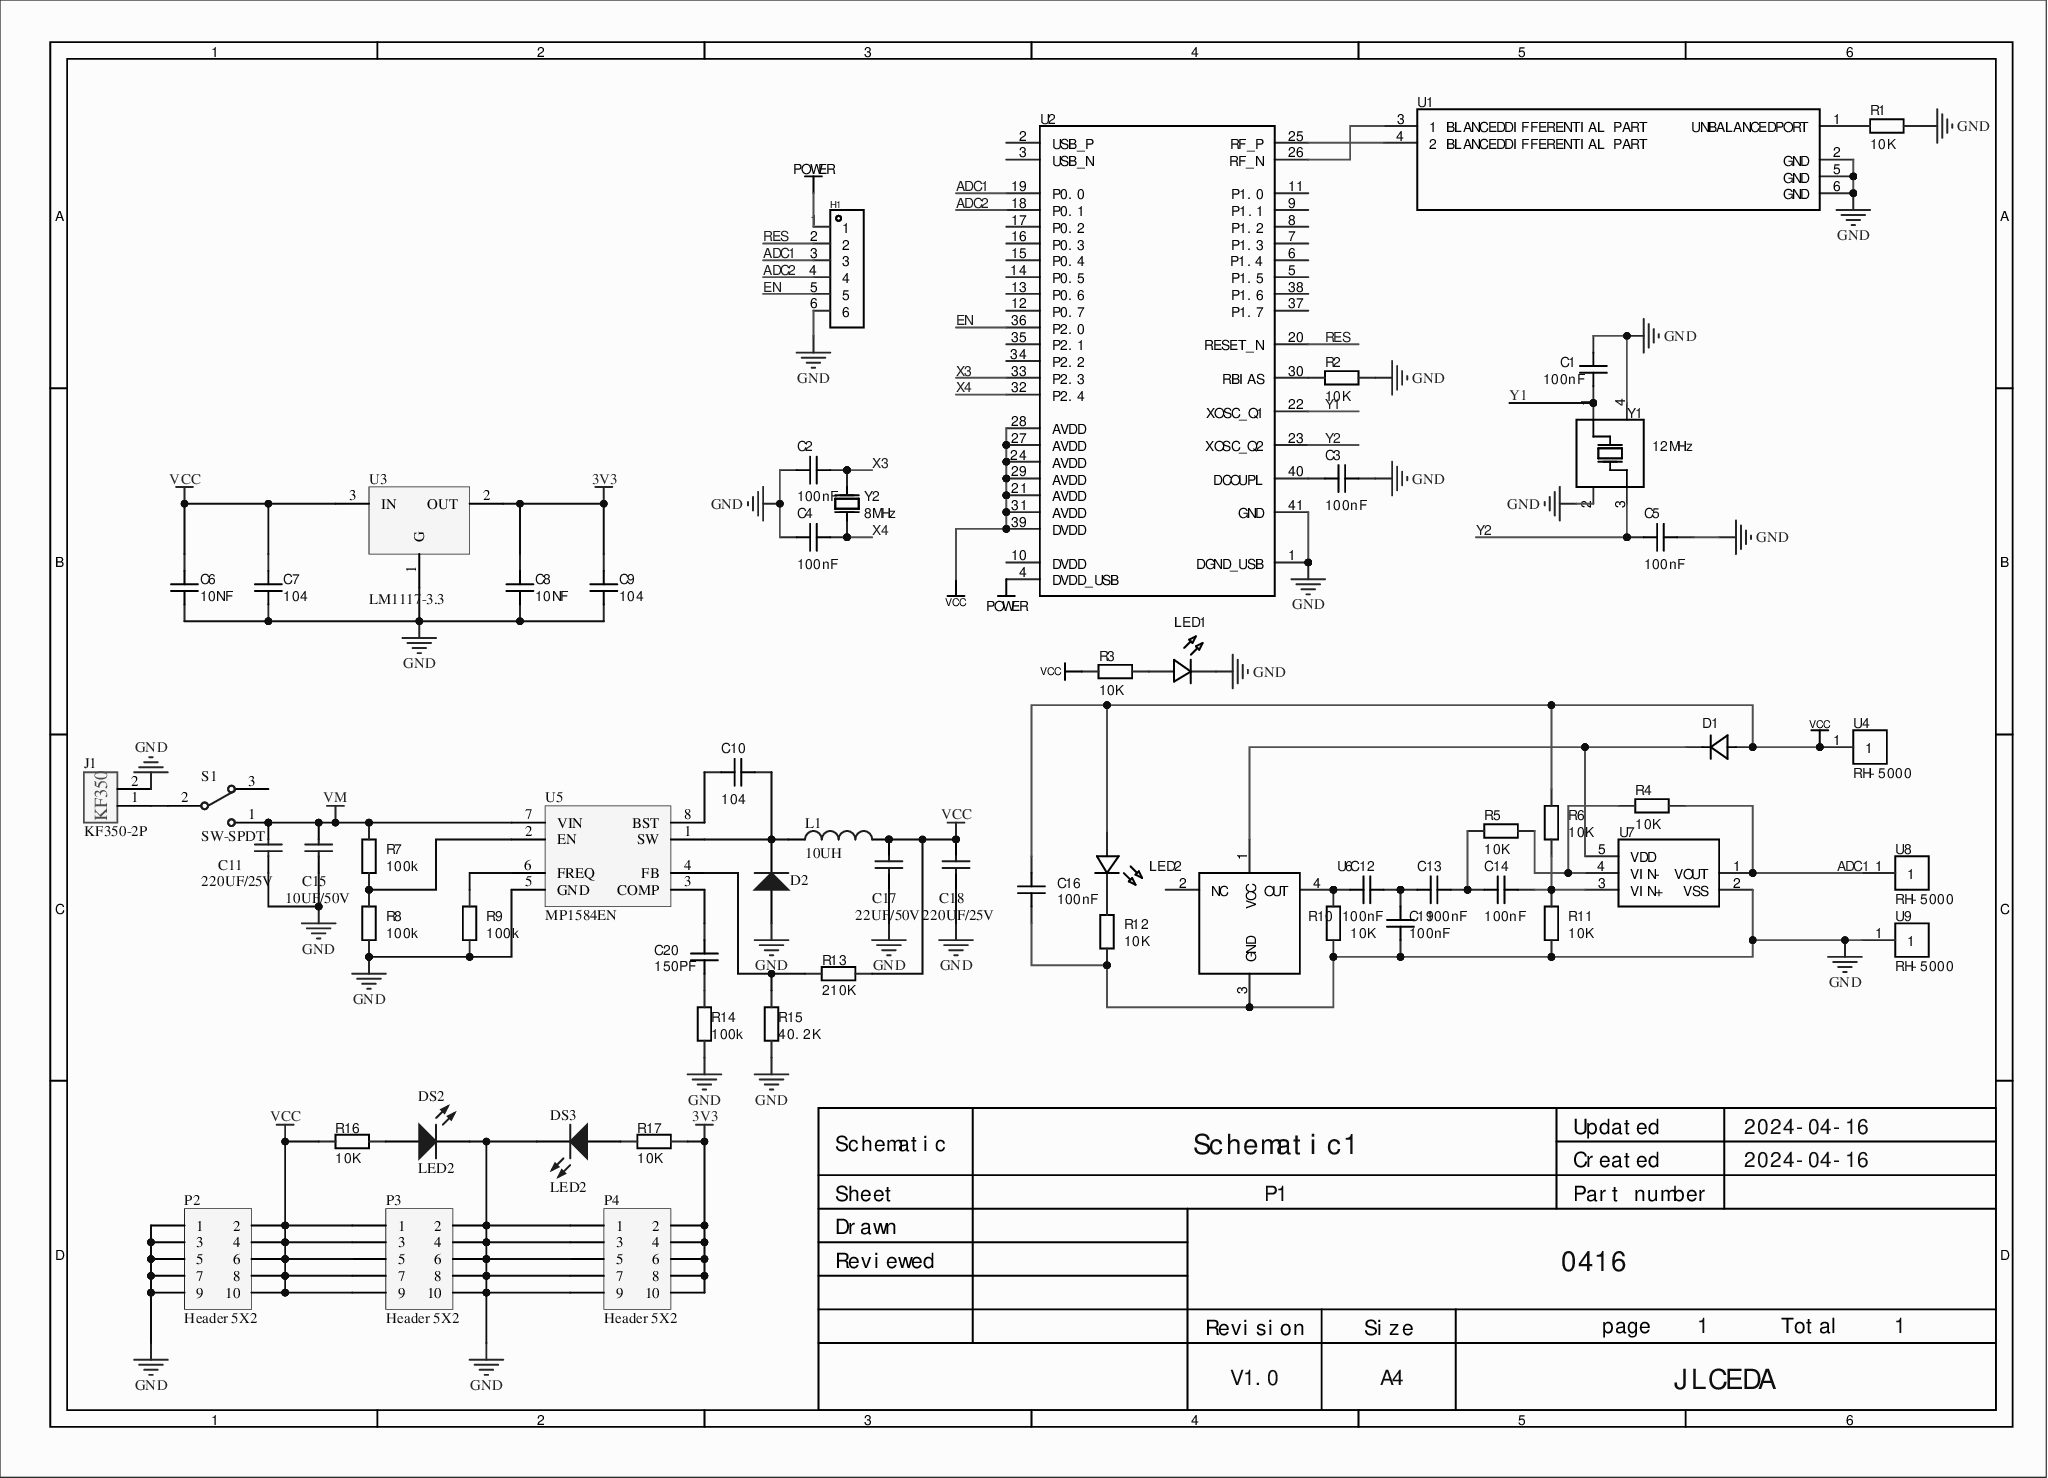
[diagram p0: MISC80555-2.SchDoc]
# Altium project MISC80555-3.PrjPcb
1 sheet, 61 parts. Net scope: global (net labels, ports and power ports of the same name join across sheets).
Board file: MISC80555.PcbDoc

## Sheet MISC80555-2.SchDoc
size 309 x 223 mm; Symbol: Sheet-Symbol_A4; Device: Sheet-Symbol_A4; @Page Name: P1; @Create Date: 2024-04-16; @Page Count: 1; @Page No: 1; @Project Name: 0416; @Schematic Name: Schematic1; @Update Date: 2024-04-16; Company: JLCEDA; Page Size: A4; Version: V1.0

### Parts
C1  100nF  [C0603]
C2  100nF  [C0603]
C3  100nF  [C0603]
C4  100nF  [C0603]
C5  100nF  [C0603]
C6  Name: 10NF  [C0603]  (hidden comment: 100nF)
C7  Name: 104  [C0603]  (hidden comment: 100nF)
C8  Name: 10NF  [C0603]  (hidden comment: 100nF)
C9  Name: 104  [C0603]  (hidden comment: 100nF)
C10  Name: 104  [C0603]  (hidden comment: 100nF)
C11  220UF/25V  [贴片电容]
C12  100nF  [C0603]
C13  100nF  [C0603]
C14  100nF  [C0603]
C15  10UF/50V  [贴片电容]
C16  100nF  [C0603]
C17  22UF/50V  [贴片电容]
C18  220UF/25V  [贴片电容]
C19  100nF  [C0603]
C20  Name: 150PF  [C0603]  (hidden comment: 100nF)
D1  D_1N4007A  [3.2X1.6X1.1]  (value not drawn)
D2  Diode BAS16  [3.2X1.6X1.1]  (value not drawn)
DS2  LED2  [my0603LED]
DS3  LED2  [my0603LED]
H1  HDR-F_2.54_1x6P  [HDR1X6]  (value not drawn)
J1  KF350-2P  [KF350-2P]
L1  10UH  [0402-A]
LED1  LED_0603-R  [my0603LED]  (value not drawn)
LED2  LED_0603-R  [my0603LED]  (value not drawn)
P2  Header 5X2  [HDR2X5]
P3  Header 5X2  [HDR2X5]
P4  Header 5X2  [HDR2X5]
R1  10K  [my0603]
R2  10K  [my0603]
R3  10K  [my0603]
R4  10K  [my0603]
R5  10K  [my0603]
R6  10K  [my0603]
R7  Name: 100k  [my0603]  (hidden comment: 10K)
R8  Name: 100k  [my0603]  (hidden comment: 10K)
R9  Name: 100k  [my0603]  (hidden comment: 10K)
R10  10K  [my0603]
R11  10K  [my0603]
R12  10K  [my0603]
R13  Name: 210K  [my0603]  (hidden comment: 10K)
R14  Name: 100k  [my0603]  (hidden comment: 10K)
R15  Name: 40.2K  [my0603]  (hidden comment: 10K)
R16  10K  [my0603]
R17  10K  [my0603]
S1  SW-SPDT  [TL36WW15050]
U1  BL1  [TSOP-6 - duplicate]  (value not drawn)
U2  CC2540  [CC254X_QFN]  (value not drawn)
U3  LM1117-3.3  [LM1117-3.3]
U4  RH-5000  [TEST-TH_BD2.54-P1.4_RED]
U5  MP1584EN  [MP1548EN]
U6  APDS  [SENSORS-SMD_APDS-9008-020]  (value not drawn)
U7  AMP  [MCP6001]  (value not drawn)
U8  RH-5000  [TEST-TH_BD2.54-P1.4_RED]
U9  RH-5000  [TEST-TH_BD2.54-P1.4_RED]
Y1  12MHz  [OSC-SMD_4P-L5.0-W3.2-BL]
Y2  8MHz  [XTAL_US]

### Nets
3V3: C8.2 C9.2 P4.2 P4.4 P4.6 P4.8 P4.10 R17.1 U3.2(OUT)
GND: C1.1 C2.1 C3.2 C4.1 C5.1 C6.1 C7.1 C8.1 C9.1 C11.1 C15.1 C16.1 C17.1 C18.1 C19.1 D2.1(A) DS2.2(K) DS3.2(K) H1.6 J1.2 LED1.1(C) P2.1 P2.3 P2.5 P2.7 P2.9 P3.2 P3.4 P3.6 P3.8 P3.10 P4.1 P4.3 P4.5 P4.7 P4.9 R1.2 R2.2 R8.1 R9.1 R10.1 R11.1 R12.1 R14.2 R15.2 U1.2(GND) U1.5(GND) U1.6(GND) U2.1(DGND_USB) U2.41(GND) U3.1(G) U5.5(GND) U6.3(GND) U7.2(VSS) U9.1 Y1.2(GND) Y1.4(GND)
POWER: H1.1 U2.4(DVDD_USB)
VCC: C6.2 C7.2 C16.2 C17.2 C18.2 D1.2(A) L1.2 LED2.2(A) P2.2 P2.4 P2.6 P2.8 P2.10 P3.1 P3.3 P3.5 P3.7 P3.9 R3.1 R6.2 R13.1 R16.2 U2.21(AVDD) U2.24(AVDD) U2.27(AVDD) U2.28(AVDD) U2.29(AVDD) U2.31(AVDD) U2.39(DVDD) U3.3(IN) U4.1
VM: C11.2 C15.2 R7.2 S1.1 U5.7(VIN)
ADC1: H1.3 R4.1 U2.19(P0.0) U7.1(VOUT) U8.1
ADC2: H1.4 U2.18(P0.1)
EN: H1.5 U2.36(P2.0)
RES: H1.2 U2.20(RESET_N)
X3: C2.2 U2.33(P2.3) Y2.1(OSC1)
X4: C4.2 U2.32(P2.4) Y2.2(OSC2)
Y1: C1.2 U2.22(XOSC_Q1) Y1.1(OSC1)
Y2: C5.2 U2.23(XOSC_Q2) Y1.3(OSC2)
NetC3_1: C3.1 U2.40(DCOUPL)
NetC10_1: C10.1 U5.8(BST)
NetC10_2: C10.2 D2.3(K) L1.1 U5.1(SW)
NetC12_1: C12.1 R10.2 U6.4(OUT)
NetC12_2: C12.2 C13.1 C19.2
NetC13_2: C13.2 C14.2 R5.1
NetC14_1: C14.1 R6.1 R11.2 U7.3(VIN+)
NetC20_1: C20.1 R14.1
NetC20_2: C20.2 U5.3(COMP)
NetD1_1: D1.1(K) U6.1(VCC) U7.5(VDD)
NetDS2_1: DS2.1(A) R16.1
NetDS3_1: DS3.1(A) R17.2
NetJ1_1: J1.1 S1.2
NetLED1_2: LED1.2(A) R3.2
NetLED2_1: LED2.1(C) R12.2
NetR1_1: R1.1 U1.1(UNBALANCEDPORT)
NetR2_1: R2.1 U2.30(RBIAS)
NetR4_2: R4.2 R5.2 U7.4(VIN-)
NetR7_1: R7.1 R8.2 U5.2(EN)
NetR9_2: R9.2 U5.6(FREQ)
NetR13_2: R13.2 R15.1 U5.4(FB)
NetU1_3: U1.3(1_BLANCEDDIFFERENTIAL_PART) U2.26(RF_N)
NetU1_4: U1.4(2_BLANCEDDIFFERENTIAL_PART) U2.25(RF_P)

Not connected (* = marked no-connect by the designer): S1 3; U2 2(USB_P) 3(USB_N) 5(P1.5) 6(P1.4) 7(P1.3) 8(P1.2) 9(P1.1) 10(DVDD) 11(P1.0) 12(P0.7) 13(P0.6) 14(P0.5) 15(P0.4) 16(P0.3) 17(P0.2) 34(P2.2) 35(P2.1) 37(P1.7) 38(P1.6); U6 2(NC)

### Notes on the sheet
- 1
- 2
- 3
- 4
- 5
- 6
- A
- B
- C
- Schematic
- Schematic1
- Created
- Updated
- 2024-04-16
- D
- Reviewed
- Drawn
- Sheet
- P1
- Part number
- 0416
- Revision
- Size
- page
- Total
- V1.0
- A4
- JLCEDA

### Library data of the parts
C1-C10 C12-C14 C16 C19 C20 = CAP_0603: Symbol: CapAcitance; Convert to PCB: yes; Device: CAP_0603; Add into BOM: yes; Supplier Footprint: 0603; Value: 100nF
  C1-C5 C12-C14 C16 C19: Name: 100nF
C11 C15 C17 C18 = Cap Semi: Capacitor (Semiconductor SIM Model); Published: 8-Jun-2000; LatestRevisionDate: 29-May-2009; LatestRevisionNote: IPC-7351 Footprint Added.; PackageReference: C1206; PackageDescription: Chip Capacitor; Publisher: Altium Limited
D1 = D_1N4007A: Add into BOM: yes; Symbol: D_1N4007; Device: D_1N4007A; Supplier Footprint: DO-41; Convert to PCB: yes
D2 = Diode BAS16: Silicon Switching Diode for High-Speed Switching; Note: Pin 2 is not connected and not drawn.; Published: 21-Mar-2003; LatestRevisionDate: 29-May-2009; LatestRevisionNote: IPC-7351 Footprint Added.; DatasheetVersion: Oct-1999; PackageVersion: Sep-2001; PackageReference: SOT-23; PackageDescription: 3-Pin SOT-23 Package 0.95 mm Pitch, 2.5 mm Lead Span; ComponentLink1Description: Manufacturer Link; ComponentLink1URL: http://www.infineon.com/; ComponentLink2Description: Datasheet; ComponentLink2URL: http://www.infineon.com/upload/Document/cmc_upload/documents/012/5331/bas16series.pdf; Publisher: Altium Limited
DS2 DS3 = LED2: Typical RED, GREEN, YELLOW, AMBER GaAs LED; Published: 8-Jun-2000; LatestRevisionDate: 17-Jul-2002; LatestRevisionNote: Re-released for DXP Platform.; PackageDocument: Feb-2002; PackageReference: 3.2X1.6X1.1; Publisher: Altium Limited
H1 = HDR-F_2.54_1x6P: Manufacturer: BOOMELE(博穆精密); Manufacturer Part: 2.54-1*6P母; Symbol: Header-Female-2.54_1x6; Convert to PCB: yes; Device: HDR-F_2.54_1x6P; Add into BOM: yes; Supplier Part: C40877; Supplier Footprint: 插件; Supplier: LCSC; JLCPCB Part Class: Extended Part
L1 = Inductor: Code_IEC: 1005; Value: 10mH; Published: 8-Jun-2000; LatestRevisionDate: 29-May-2009; LatestRevisionNote: IPC-7351 Footprint Added.; PackageReference: 0402-A; PackageDescription: Chip Inductor; Code_JEITA: 0402; Publisher: Altium Limited
LED1 LED2 = LED_0603-R: Symbol: LED_R; Convert to PCB: yes; Device: LED_0603-R; Add into BOM: yes; Supplier Footprint: 0603
P2-P4 = Header 5X2: Header, 5-Pin, Dual row; LatestRevisionDate: 17-Jul-2002; LatestRevisionNote: Re-released for DXP Platform.; Publisher: Altium Limited
R1-R17 = Res_0603: Symbol: Resistor; Convert to PCB: yes; Device: Res_0603; Add into BOM: yes; Supplier Footprint: 0603; Value: 10K
  R1-R6 R10-R12 R16 R17: Name: 10K
S1 = SW-SPDT: SPDT Subminiature Toggle Switch, Right Angle Mounting, Vertical Actuation; Published: 24-Mar-1999; LatestRevisionDate: 17-Dec-2003; LatestRevisionNote: Schematic revised, PCB Footprint replaced.; DatasheetVersion: 05-Dec-2000; PackageReference: TL36WW15050; PackageDescription: Switch; 4 Leads; ComponentLink1Description: Manufacturer Link; ComponentLink1URL: http://www.apem.com; Publisher: Altium Limited
U1 = BL1: Add into BOM: yes; Symbol: BL1; Device: BL1; Convert to PCB: yes
U2 = CC2540: Add into BOM: yes; Symbol: CC2540; Device: CC2540; Convert to PCB: yes
U3 = LM1117: LINER REG
U4 U8 U9 = RH-5000: Manufacturer: 荣和; Add into BOM: yes; Name: RH-5000; Symbol: RH-5000; Device: RH-5000; LCSC Part Name: PCB电路板测试点/测试针; Supplier Part: C5277086; Manufacturer Part: RH-5000; Supplier Footprint: -; JLCPCB Part Class: Extended library; Datasheet: https://atta.szlcsc.com/upload/public/pdf/source/20230704/1671C2774A3D6CEDC1FD6AAF48538C87.pdf; Supplier: LCSC; Convert to PCB: yes
U6 = APDS: Add into BOM: yes; Symbol: APDS; Device: APDS; Convert to PCB: yes
U7 = AMP: Add into BOM: yes; Symbol: AMP; Device: AMP; Convert to PCB: yes
Y1 = X322512MSB4SI: Crystal type: SMD crystal; frequency: 12MHz; frequency tolerance (room temp): ±10ppm; load capacitance: 20pF; frequency stability (full temp): ±20ppm;; Manufacturer: YXC(扬兴晶振); Add into BOM: yes; Name: 12MHz; Symbol: X322512MSB4SI; Device: X322512MSB4SI; LCSC Part Name: 12MHz ±10ppm 20pF; Supplier Part: C9002; Manufacturer Part: X322512MSB4SI; Supplier Footprint: SMD3225-4P; JLCPCB Part Class: Basic library; Datasheet: https://atta.szlcsc.com/upload/public/pdf/source/20240329/19D5F850207469550BEB00D7DFEDBC7A.pdf; Supplier: LCSC; Convert to PCB: yes; Crystal Type: SMD crystal; Value: 12MHz; Normal temperature Frequency Tolerance: ±10ppm; External load capacitor: 20pF; Frequency Stability(Full temperature range): ±20ppm; Operating Temperature: -40℃~+85℃
Y2 = X49SM8MSD2SC: Crystal type: SMD crystal; frequency: 8MHz; frequency tolerance (room temp): ±20ppm; load capacitance: 20pF; frequency stability (full temp): ±30ppm;; Manufacturer: YXC(扬兴晶振); Add into BOM: yes; Name: 8MHz; Symbol: X49SM8MSD2SC; Device: X49SM8MSD2SC; LCSC Part Name: 8MHz ±20ppm 20pF; Supplier Part: C12674; Manufacturer Part: X49SM8MSD2SC; Supplier Footprint: HC-49S-SMD; JLCPCB Part Class: Basic library; Datasheet: https://atta.szlcsc.com/upload/public/pdf/source/20240329/3EBF42EBCAB50CA65B6FA9D7CFA1955A.pdf; Supplier: LCSC; Convert to PCB: yes; Crystal Type: SMD crystal; Value: 8MHz; Normal temperature Frequency Tolerance: ±20ppm; External load capacitor: 20pF; Frequency Stability(Full temperature range): ±30ppm; Operating Temperature: -20℃~+70℃